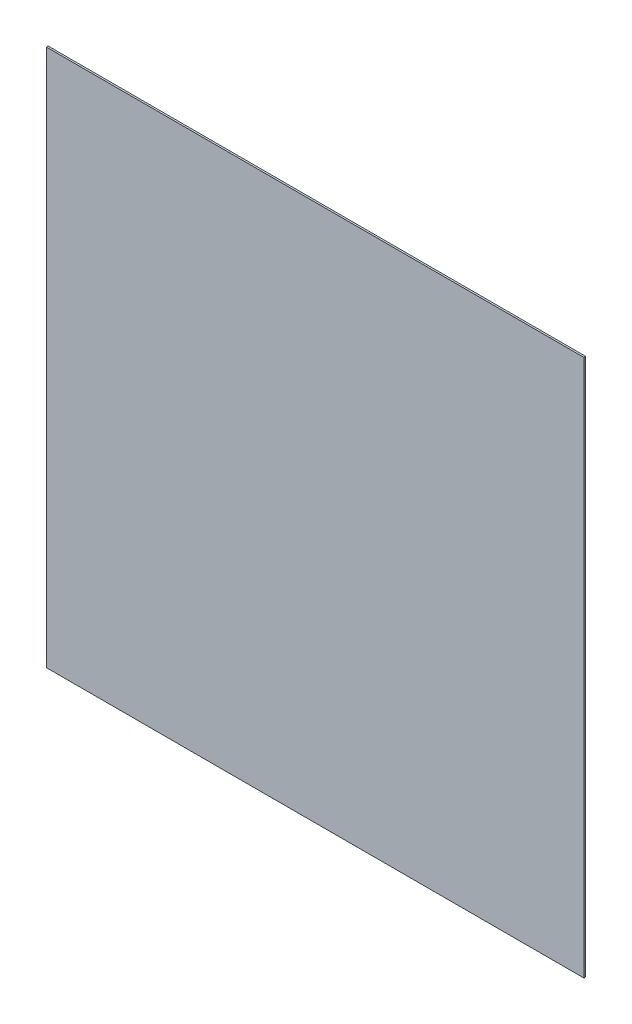
SolidWorks part; units mm, degrees
ref_plane "前视基准面" through (0, 0, 0) normal (0, 0, 1) x (1, 0, 0)
ref_plane "上视基准面" through (0, 0, 0) normal (0, 1, 0) x (1, 0, 0)
ref_plane "右视基准面" through (0, 0, 0) normal (1, 0, 0) x (0, 0, -1)
sketch "草图1" plane through (0, 0, 0) normal (0, 0, 1) x (1, 0, 0)
  line L1 (-300, 300) -> (300, 300)
  line L2 (-300, 300) -> (-300, -300)
  line L3 (-300, -300) -> (300, -300)
  line L4 (300, 300) -> (300, -300)
  line L5 (-300, 300) -> (300, -300) construction
  line L6 (-300, -300) -> (300, 300) construction
  point P0 (0, 0)
  dimension "D1" = 600
extrude "凸台-拉伸1" add sketch "草图1" along normal blind 2
